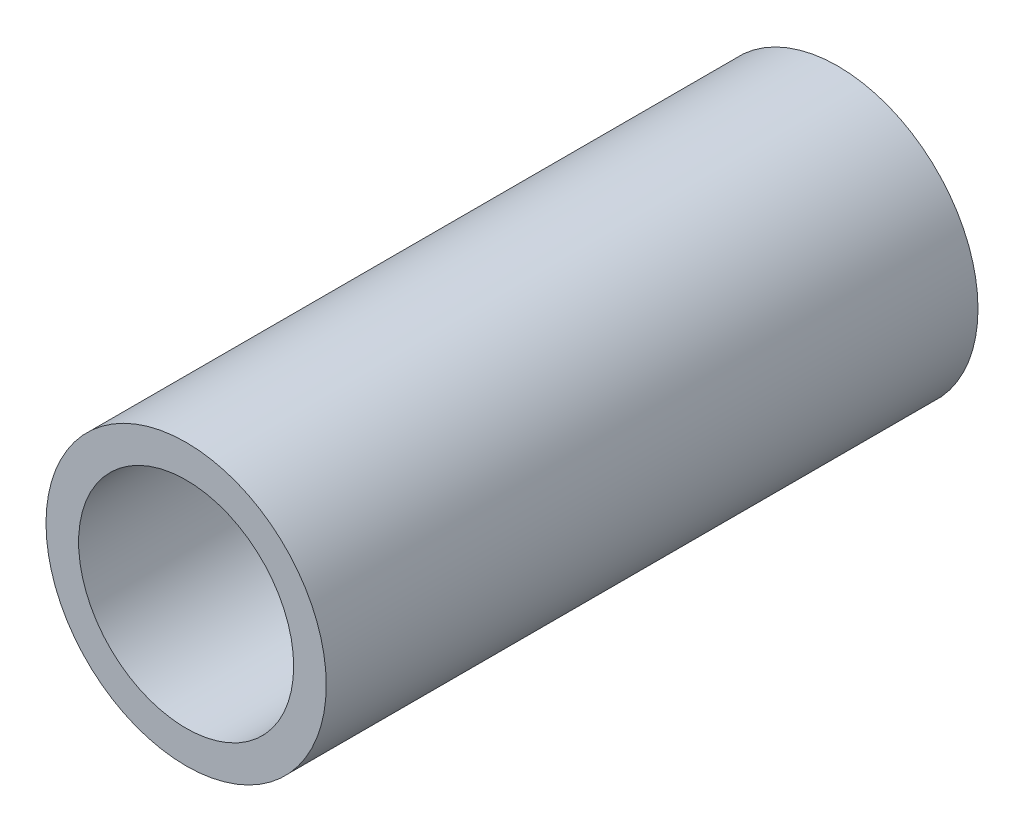
from build123d import *

# Parameters (mm, degrees)
SKETCH_1_R      = 21.5
SKETCH_1_R_2    = 16.5
EXTRUDE_1_DEPTH = 100


with BuildPart() as part:
    # 草图1 → 凸台-拉伸1 (new body)
    with BuildSketch(Plane.XY):
        Circle(SKETCH_1_R)
        Circle(SKETCH_1_R_2, mode=Mode.SUBTRACT)
    extrude(amount=EXTRUDE_1_DEPTH)


solid = part.part
